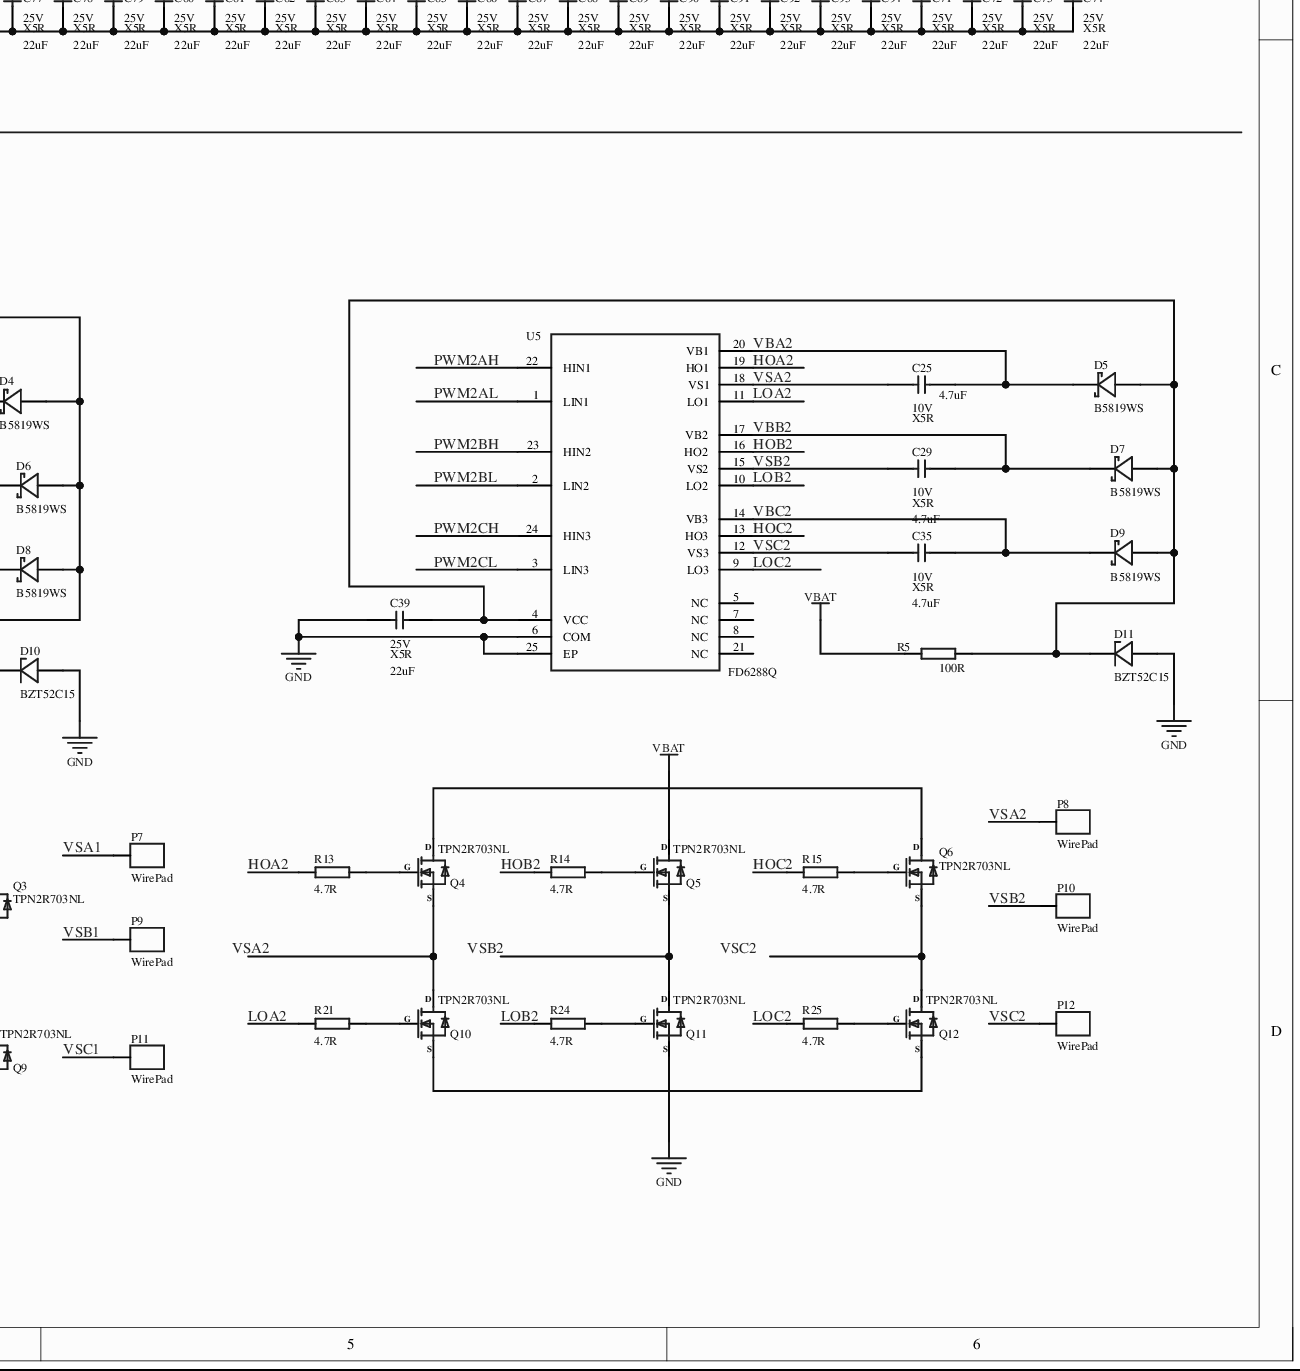
[diagram p0: MISC49862-3.schdoc, bottom right]
# Altium project MISC49862-2.PrjPcb (part 4 of 4)

## Sheet MISC49862-3.schdoc (continued)

### Library data of the parts (continued)
R9 = =Value+' '+Tolerance: SMD resistor; Device: 100R ±1%; Symbol: Res-Chip; Tolerance: ±1%; Origin Footprint 2: RESC0603[0201]-L; Origin Footprint 3: RESC0603[0201]-M; Origin Footprint 4: RESC0603[0201]-N; Origin Footprint 5: RESC0603[0201]S-L; Origin Footprint 6: RESC0603[0201]S-M; Origin Footprint 7: RESC0603[0201]S-N; Origin Footprint 8: RESC1005[0402]-L; Origin Footprint 9: RESC1005[0402]-M; Origin Footprint 10: RESC1005[0402]-N; Origin Footprint 11: RESC1005[0402]S-L; Origin Footprint 12: RESC1005[0402]S-M; Origin Footprint 13: RESC1608[0603]-L; Origin Footprint 14: RESC1608[0603]-M; Origin Footprint 15: RESC1608[0603]-N; Origin Footprint 16: RESC1608[0603]S-L; Origin Footprint 17: RESC1608[0603]S-M; Origin Footprint 18: RESC1608[0603]S-N; Origin Footprint 19: RESC2012[0805]; Origin Footprint 20: RESC2012[0805]S-L; Origin Footprint 21: RESC2012[0805]S-M; Origin Footprint 22: RESC2012[0805]S-N; Origin Footprint 23: RESC3216[1206]; Origin Footprint 24: RESC3216[1206]S-L; Origin Footprint 25: RESC3216[1206]S-M; Origin Footprint 26: RESC3216[1206]S-N; Origin Footprint 27: RESC3225[1210]; Origin Footprint 28: RESC3225[1210]S; Origin Footprint 29: RESC5025[2010]; Origin Footprint 30: RESC5025[2010]S; Origin Footprint 31: RESC6332[2512]; Origin Footprint 32: RESC6332[2512]S; UniqueId: 1e1ffada38203b9e; AddInBom: yes; Origin Footprint 1: RESC1005[0402]S-N; Design Item ID: Res-Chip; Library Name: Brushless driver-CYT2BL3-FD6288-FOC-LiteDual; Revision: V1.0; FootprintName: RESC1005[0402]S-N; ConvertToPcb: yes
R10 = =Value+' '+Tolerance: SMD resistor; Device: 4.7K ±1%; Symbol: Res-Chip_4; Tolerance: ±1%; Origin Footprint 2: RESC0603[0201]-L; Origin Footprint 3: RESC0603[0201]-M; Origin Footprint 4: RESC0603[0201]-N; Origin Footprint 5: RESC0603[0201]S-L; Origin Footprint 6: RESC0603[0201]S-M; Origin Footprint 7: RESC0603[0201]S-N; Origin Footprint 8: RESC1005[0402]-L; Origin Footprint 9: RESC1005[0402]-M; Origin Footprint 10: RESC1005[0402]-N; Origin Footprint 11: RESC1005[0402]S-L; Origin Footprint 12: RESC1005[0402]S-M; Origin Footprint 13: RESC1608[0603]-L; Origin Footprint 14: RESC1608[0603]-M; Origin Footprint 15: RESC1608[0603]-N; Origin Footprint 16: RESC1608[0603]S-L; Origin Footprint 17: RESC1608[0603]S-M; Origin Footprint 18: RESC1608[0603]S-N; Origin Footprint 19: RESC2012[0805]; Origin Footprint 20: RESC2012[0805]S-L; Origin Footprint 21: RESC2012[0805]S-M; Origin Footprint 22: RESC2012[0805]S-N; Origin Footprint 23: RESC3216[1206]; Origin Footprint 24: RESC3216[1206]S-L; Origin Footprint 25: RESC3216[1206]S-M; Origin Footprint 26: RESC3216[1206]S-N; Origin Footprint 27: RESC3225[1210]; Origin Footprint 28: RESC3225[1210]S; Origin Footprint 29: RESC5025[2010]; Origin Footprint 30: RESC5025[2010]S; Origin Footprint 31: RESC6332[2512]; Origin Footprint 32: RESC6332[2512]S; UniqueId: 41bc0941336b1513; AddInBom: yes; Origin Footprint 1: RESC1005[0402]S-N; Design Item ID: Res-Chip_4; Library Name: Brushless driver-CYT2BL3-FD6288-FOC-LiteDual; Revision: V1.0; FootprintName: RESC1005[0402]S-N; ConvertToPcb: yes
R11 = =Value+' '+Tolerance: SMD resistor; Device: 4.7R ±1%; Symbol: Res-Chip_7; Tolerance: ±1%; Origin Footprint 2: RESC0603[0201]-L; Origin Footprint 3: RESC0603[0201]-M; Origin Footprint 4: RESC0603[0201]-N; Origin Footprint 5: RESC0603[0201]S-L; Origin Footprint 6: RESC0603[0201]S-M; Origin Footprint 7: RESC0603[0201]S-N; Origin Footprint 8: RESC1005[0402]-L; Origin Footprint 9: RESC1005[0402]-M; Origin Footprint 10: RESC1005[0402]-N; Origin Footprint 11: RESC1005[0402]S-L; Origin Footprint 12: RESC1005[0402]S-M; Origin Footprint 13: RESC1608[0603]-L; Origin Footprint 14: RESC1608[0603]-M; Origin Footprint 15: RESC1608[0603]-N; Origin Footprint 16: RESC1608[0603]S-L; Origin Footprint 17: RESC1608[0603]S-M; Origin Footprint 18: RESC1608[0603]S-N; Origin Footprint 19: RESC2012[0805]; Origin Footprint 20: RESC2012[0805]S-L; Origin Footprint 21: RESC2012[0805]S-M; Origin Footprint 22: RESC2012[0805]S-N; Origin Footprint 23: RESC3216[1206]; Origin Footprint 24: RESC3216[1206]S-L; Origin Footprint 25: RESC3216[1206]S-M; Origin Footprint 26: RESC3216[1206]S-N; Origin Footprint 27: RESC3225[1210]; Origin Footprint 28: RESC3225[1210]S; Origin Footprint 29: RESC5025[2010]; Origin Footprint 30: RESC5025[2010]S; Origin Footprint 31: RESC6332[2512]; Origin Footprint 32: RESC6332[2512]S; UniqueId: 763cf8d5648cb4fd; AddInBom: yes; Origin Footprint 1: RESC1005[0402]S-N; Design Item ID: Res-Chip; Library Name: SEEKFREE_Device; Revision: V1.0; FootprintName: RESC1005[0402]S-N; ConvertToPcb: yes
R12 = =Value+' '+Tolerance: SMD resistor; Device: 1K ±1%; Symbol: Res-Chip_3; Tolerance: ±1%; Origin Footprint 2: RESC0603[0201]-L; Origin Footprint 3: RESC0603[0201]-M; Origin Footprint 4: RESC0603[0201]-N; Origin Footprint 5: RESC0603[0201]S-L; Origin Footprint 6: RESC0603[0201]S-M; Origin Footprint 7: RESC0603[0201]S-N; Origin Footprint 8: RESC1005[0402]-L; Origin Footprint 9: RESC1005[0402]-M; Origin Footprint 10: RESC1005[0402]-N; Origin Footprint 11: RESC1005[0402]S-L; Origin Footprint 12: RESC1005[0402]S-M; Origin Footprint 13: RESC1608[0603]-L; Origin Footprint 14: RESC1608[0603]-M; Origin Footprint 15: RESC1608[0603]-N; Origin Footprint 16: RESC1608[0603]S-L; Origin Footprint 17: RESC1608[0603]S-M; Origin Footprint 18: RESC1608[0603]S-N; Origin Footprint 19: RESC2012[0805]; Origin Footprint 20: RESC2012[0805]S-L; Origin Footprint 21: RESC2012[0805]S-M; Origin Footprint 22: RESC2012[0805]S-N; Origin Footprint 23: RESC3216[1206]; Origin Footprint 24: RESC3216[1206]S-L; Origin Footprint 25: RESC3216[1206]S-M; Origin Footprint 26: RESC3216[1206]S-N; Origin Footprint 27: RESC3225[1210]; Origin Footprint 28: RESC3225[1210]S; Origin Footprint 29: RESC5025[2010]; Origin Footprint 30: RESC5025[2010]S; Origin Footprint 31: RESC6332[2512]; Origin Footprint 32: RESC6332[2512]S; UniqueId: 15ac9218146e0f4b; AddInBom: yes; Origin Footprint 1: RESC1005[0402]S-N; Design Item ID: Res-Chip_3; Library Name: Brushless driver-CYT2BL3-FD6288-FOC-LiteDual; Revision: V1.0; FootprintName: RESC1005[0402]S-N; ConvertToPcb: yes
R13 = =Value+' '+Tolerance: SMD resistor; Device: 4.7R ±1%; Symbol: Res-Chip_7; Tolerance: ±1%; Origin Footprint 2: RESC0603[0201]-L; Origin Footprint 3: RESC0603[0201]-M; Origin Footprint 4: RESC0603[0201]-N; Origin Footprint 5: RESC0603[0201]S-L; Origin Footprint 6: RESC0603[0201]S-M; Origin Footprint 7: RESC0603[0201]S-N; Origin Footprint 8: RESC1005[0402]-L; Origin Footprint 9: RESC1005[0402]-M; Origin Footprint 10: RESC1005[0402]-N; Origin Footprint 11: RESC1005[0402]S-L; Origin Footprint 12: RESC1005[0402]S-M; Origin Footprint 13: RESC1608[0603]-L; Origin Footprint 14: RESC1608[0603]-M; Origin Footprint 15: RESC1608[0603]-N; Origin Footprint 16: RESC1608[0603]S-L; Origin Footprint 17: RESC1608[0603]S-M; Origin Footprint 18: RESC1608[0603]S-N; Origin Footprint 19: RESC2012[0805]; Origin Footprint 20: RESC2012[0805]S-L; Origin Footprint 21: RESC2012[0805]S-M; Origin Footprint 22: RESC2012[0805]S-N; Origin Footprint 23: RESC3216[1206]; Origin Footprint 24: RESC3216[1206]S-L; Origin Footprint 25: RESC3216[1206]S-M; Origin Footprint 26: RESC3216[1206]S-N; Origin Footprint 27: RESC3225[1210]; Origin Footprint 28: RESC3225[1210]S; Origin Footprint 29: RESC5025[2010]; Origin Footprint 30: RESC5025[2010]S; Origin Footprint 31: RESC6332[2512]; Origin Footprint 32: RESC6332[2512]S; UniqueId: ff4077a9ca69db92; AddInBom: yes; Origin Footprint 1: RESC1005[0402]S-N; Design Item ID: Res-Chip; Library Name: SEEKFREE_Device; Revision: V1.0; FootprintName: RESC1005[0402]S-N; ConvertToPcb: yes
R14 = =Value+' '+Tolerance: SMD resistor; Device: 4.7R ±1%; Symbol: Res-Chip_7; Tolerance: ±1%; Origin Footprint 2: RESC0603[0201]-L; Origin Footprint 3: RESC0603[0201]-M; Origin Footprint 4: RESC0603[0201]-N; Origin Footprint 5: RESC0603[0201]S-L; Origin Footprint 6: RESC0603[0201]S-M; Origin Footprint 7: RESC0603[0201]S-N; Origin Footprint 8: RESC1005[0402]-L; Origin Footprint 9: RESC1005[0402]-M; Origin Footprint 10: RESC1005[0402]-N; Origin Footprint 11: RESC1005[0402]S-L; Origin Footprint 12: RESC1005[0402]S-M; Origin Footprint 13: RESC1608[0603]-L; Origin Footprint 14: RESC1608[0603]-M; Origin Footprint 15: RESC1608[0603]-N; Origin Footprint 16: RESC1608[0603]S-L; Origin Footprint 17: RESC1608[0603]S-M; Origin Footprint 18: RESC1608[0603]S-N; Origin Footprint 19: RESC2012[0805]; Origin Footprint 20: RESC2012[0805]S-L; Origin Footprint 21: RESC2012[0805]S-M; Origin Footprint 22: RESC2012[0805]S-N; Origin Footprint 23: RESC3216[1206]; Origin Footprint 24: RESC3216[1206]S-L; Origin Footprint 25: RESC3216[1206]S-M; Origin Footprint 26: RESC3216[1206]S-N; Origin Footprint 27: RESC3225[1210]; Origin Footprint 28: RESC3225[1210]S; Origin Footprint 29: RESC5025[2010]; Origin Footprint 30: RESC5025[2010]S; Origin Footprint 31: RESC6332[2512]; Origin Footprint 32: RESC6332[2512]S; UniqueId: 8b54177fc4d64d35; AddInBom: yes; Origin Footprint 1: RESC1005[0402]S-N; Design Item ID: Res-Chip; Library Name: SEEKFREE_Device; Revision: V1.0; FootprintName: RESC1005[0402]S-N; ConvertToPcb: yes
R15 = =Value+' '+Tolerance: SMD resistor; Device: 4.7R ±1%; Symbol: Res-Chip_7; Tolerance: ±1%; Origin Footprint 2: RESC0603[0201]-L; Origin Footprint 3: RESC0603[0201]-M; Origin Footprint 4: RESC0603[0201]-N; Origin Footprint 5: RESC0603[0201]S-L; Origin Footprint 6: RESC0603[0201]S-M; Origin Footprint 7: RESC0603[0201]S-N; Origin Footprint 8: RESC1005[0402]-L; Origin Footprint 9: RESC1005[0402]-M; Origin Footprint 10: RESC1005[0402]-N; Origin Footprint 11: RESC1005[0402]S-L; Origin Footprint 12: RESC1005[0402]S-M; Origin Footprint 13: RESC1608[0603]-L; Origin Footprint 14: RESC1608[0603]-M; Origin Footprint 15: RESC1608[0603]-N; Origin Footprint 16: RESC1608[0603]S-L; Origin Footprint 17: RESC1608[0603]S-M; Origin Footprint 18: RESC1608[0603]S-N; Origin Footprint 19: RESC2012[0805]; Origin Footprint 20: RESC2012[0805]S-L; Origin Footprint 21: RESC2012[0805]S-M; Origin Footprint 22: RESC2012[0805]S-N; Origin Footprint 23: RESC3216[1206]; Origin Footprint 24: RESC3216[1206]S-L; Origin Footprint 25: RESC3216[1206]S-M; Origin Footprint 26: RESC3216[1206]S-N; Origin Footprint 27: RESC3225[1210]; Origin Footprint 28: RESC3225[1210]S; Origin Footprint 29: RESC5025[2010]; Origin Footprint 30: RESC5025[2010]S; Origin Footprint 31: RESC6332[2512]; Origin Footprint 32: RESC6332[2512]S; UniqueId: feece054417b9159; AddInBom: yes; Origin Footprint 1: RESC1005[0402]S-N; Design Item ID: Res-Chip; Library Name: SEEKFREE_Device; Revision: V1.0; FootprintName: RESC1005[0402]S-N; ConvertToPcb: yes
R16 = =Value+' '+Tolerance: SMD resistor; Device: 4.7R ±1%; Symbol: Res-Chip_7; Tolerance: ±1%; Origin Footprint 2: RESC0603[0201]-L; Origin Footprint 3: RESC0603[0201]-M; Origin Footprint 4: RESC0603[0201]-N; Origin Footprint 5: RESC0603[0201]S-L; Origin Footprint 6: RESC0603[0201]S-M; Origin Footprint 7: RESC0603[0201]S-N; Origin Footprint 8: RESC1005[0402]-L; Origin Footprint 9: RESC1005[0402]-M; Origin Footprint 10: RESC1005[0402]-N; Origin Footprint 11: RESC1005[0402]S-L; Origin Footprint 12: RESC1005[0402]S-M; Origin Footprint 13: RESC1608[0603]-L; Origin Footprint 14: RESC1608[0603]-M; Origin Footprint 15: RESC1608[0603]-N; Origin Footprint 16: RESC1608[0603]S-L; Origin Footprint 17: RESC1608[0603]S-M; Origin Footprint 18: RESC1608[0603]S-N; Origin Footprint 19: RESC2012[0805]; Origin Footprint 20: RESC2012[0805]S-L; Origin Footprint 21: RESC2012[0805]S-M; Origin Footprint 22: RESC2012[0805]S-N; Origin Footprint 23: RESC3216[1206]; Origin Footprint 24: RESC3216[1206]S-L; Origin Footprint 25: RESC3216[1206]S-M; Origin Footprint 26: RESC3216[1206]S-N; Origin Footprint 27: RESC3225[1210]; Origin Footprint 28: RESC3225[1210]S; Origin Footprint 29: RESC5025[2010]; Origin Footprint 30: RESC5025[2010]S; Origin Footprint 31: RESC6332[2512]; Origin Footprint 32: RESC6332[2512]S; UniqueId: 3c543c7c58e1cc80; AddInBom: yes; Origin Footprint 1: RESC1005[0402]S-N; Design Item ID: Res-Chip; Library Name: SEEKFREE_Device; Revision: V1.0; FootprintName: RESC1005[0402]S-N; ConvertToPcb: yes
R17 = =Value+' '+Tolerance: SMD resistor; Device: 1K ±1%; Symbol: Res-Chip_3; Tolerance: ±1%; Origin Footprint 2: RESC0603[0201]-L; Origin Footprint 3: RESC0603[0201]-M; Origin Footprint 4: RESC0603[0201]-N; Origin Footprint 5: RESC0603[0201]S-L; Origin Footprint 6: RESC0603[0201]S-M; Origin Footprint 7: RESC0603[0201]S-N; Origin Footprint 8: RESC1005[0402]-L; Origin Footprint 9: RESC1005[0402]-M; Origin Footprint 10: RESC1005[0402]-N; Origin Footprint 11: RESC1005[0402]S-L; Origin Footprint 12: RESC1005[0402]S-M; Origin Footprint 13: RESC1608[0603]-L; Origin Footprint 14: RESC1608[0603]-M; Origin Footprint 15: RESC1608[0603]-N; Origin Footprint 16: RESC1608[0603]S-L; Origin Footprint 17: RESC1608[0603]S-M; Origin Footprint 18: RESC1608[0603]S-N; Origin Footprint 19: RESC2012[0805]; Origin Footprint 20: RESC2012[0805]S-L; Origin Footprint 21: RESC2012[0805]S-M; Origin Footprint 22: RESC2012[0805]S-N; Origin Footprint 23: RESC3216[1206]; Origin Footprint 24: RESC3216[1206]S-L; Origin Footprint 25: RESC3216[1206]S-M; Origin Footprint 26: RESC3216[1206]S-N; Origin Footprint 27: RESC3225[1210]; Origin Footprint 28: RESC3225[1210]S; Origin Footprint 29: RESC5025[2010]; Origin Footprint 30: RESC5025[2010]S; Origin Footprint 31: RESC6332[2512]; Origin Footprint 32: RESC6332[2512]S; UniqueId: 6346d187b4e0bc9c; AddInBom: yes; Origin Footprint 1: RESC1005[0402]S-N; Design Item ID: Res-Chip_3; Library Name: Brushless driver-CYT2BL3-FD6288-FOC-LiteDual; Revision: V1.0; FootprintName: RESC1005[0402]S-N; ConvertToPcb: yes
R18 = =Value+' '+Tolerance: SMD resistor; Device: 4.7R ±1%; Symbol: Res-Chip_7; Tolerance: ±1%; Origin Footprint 2: RESC0603[0201]-L; Origin Footprint 3: RESC0603[0201]-M; Origin Footprint 4: RESC0603[0201]-N; Origin Footprint 5: RESC0603[0201]S-L; Origin Footprint 6: RESC0603[0201]S-M; Origin Footprint 7: RESC0603[0201]S-N; Origin Footprint 8: RESC1005[0402]-L; Origin Footprint 9: RESC1005[0402]-M; Origin Footprint 10: RESC1005[0402]-N; Origin Footprint 11: RESC1005[0402]S-L; Origin Footprint 12: RESC1005[0402]S-M; Origin Footprint 13: RESC1608[0603]-L; Origin Footprint 14: RESC1608[0603]-M; Origin Footprint 15: RESC1608[0603]-N; Origin Footprint 16: RESC1608[0603]S-L; Origin Footprint 17: RESC1608[0603]S-M; Origin Footprint 18: RESC1608[0603]S-N; Origin Footprint 19: RESC2012[0805]; Origin Footprint 20: RESC2012[0805]S-L; Origin Footprint 21: RESC2012[0805]S-M; Origin Footprint 22: RESC2012[0805]S-N; Origin Footprint 23: RESC3216[1206]; Origin Footprint 24: RESC3216[1206]S-L; Origin Footprint 25: RESC3216[1206]S-M; Origin Footprint 26: RESC3216[1206]S-N; Origin Footprint 27: RESC3225[1210]; Origin Footprint 28: RESC3225[1210]S; Origin Footprint 29: RESC5025[2010]; Origin Footprint 30: RESC5025[2010]S; Origin Footprint 31: RESC6332[2512]; Origin Footprint 32: RESC6332[2512]S; UniqueId: 5f673669f0d56d8f; AddInBom: yes; Origin Footprint 1: RESC1005[0402]S-N; Design Item ID: Res-Chip; Library Name: SEEKFREE_Device; Revision: V1.0; FootprintName: RESC1005[0402]S-N; ConvertToPcb: yes
R19 = =Value+' '+Tolerance: SMD resistor; Device: 4.7R ±1%; Symbol: Res-Chip_7; Tolerance: ±1%; Origin Footprint 2: RESC0603[0201]-L; Origin Footprint 3: RESC0603[0201]-M; Origin Footprint 4: RESC0603[0201]-N; Origin Footprint 5: RESC0603[0201]S-L; Origin Footprint 6: RESC0603[0201]S-M; Origin Footprint 7: RESC0603[0201]S-N; Origin Footprint 8: RESC1005[0402]-L; Origin Footprint 9: RESC1005[0402]-M; Origin Footprint 10: RESC1005[0402]-N; Origin Footprint 11: RESC1005[0402]S-L; Origin Footprint 12: RESC1005[0402]S-M; Origin Footprint 13: RESC1608[0603]-L; Origin Footprint 14: RESC1608[0603]-M; Origin Footprint 15: RESC1608[0603]-N; Origin Footprint 16: RESC1608[0603]S-L; Origin Footprint 17: RESC1608[0603]S-M; Origin Footprint 18: RESC1608[0603]S-N; Origin Footprint 19: RESC2012[0805]; Origin Footprint 20: RESC2012[0805]S-L; Origin Footprint 21: RESC2012[0805]S-M; Origin Footprint 22: RESC2012[0805]S-N; Origin Footprint 23: RESC3216[1206]; Origin Footprint 24: RESC3216[1206]S-L; Origin Footprint 25: RESC3216[1206]S-M; Origin Footprint 26: RESC3216[1206]S-N; Origin Footprint 27: RESC3225[1210]; Origin Footprint 28: RESC3225[1210]S; Origin Footprint 29: RESC5025[2010]; Origin Footprint 30: RESC5025[2010]S; Origin Footprint 31: RESC6332[2512]; Origin Footprint 32: RESC6332[2512]S; UniqueId: a32210a39874d8f8; AddInBom: yes; Origin Footprint 1: RESC1005[0402]S-N; Design Item ID: Res-Chip; Library Name: SEEKFREE_Device; Revision: V1.0; FootprintName: RESC1005[0402]S-N; ConvertToPcb: yes
R20 = =Value+' '+Tolerance: SMD resistor; Device: 100R ±1%; Symbol: Res-Chip; Tolerance: ±1%; Origin Footprint 2: RESC0603[0201]-L; Origin Footprint 3: RESC0603[0201]-M; Origin Footprint 4: RESC0603[0201]-N; Origin Footprint 5: RESC0603[0201]S-L; Origin Footprint 6: RESC0603[0201]S-M; Origin Footprint 7: RESC0603[0201]S-N; Origin Footprint 8: RESC1005[0402]-L; Origin Footprint 9: RESC1005[0402]-M; Origin Footprint 10: RESC1005[0402]-N; Origin Footprint 11: RESC1005[0402]S-L; Origin Footprint 12: RESC1005[0402]S-M; Origin Footprint 13: RESC1608[0603]-L; Origin Footprint 14: RESC1608[0603]-M; Origin Footprint 15: RESC1608[0603]-N; Origin Footprint 16: RESC1608[0603]S-L; Origin Footprint 17: RESC1608[0603]S-M; Origin Footprint 18: RESC1608[0603]S-N; Origin Footprint 19: RESC2012[0805]; Origin Footprint 20: RESC2012[0805]S-L; Origin Footprint 21: RESC2012[0805]S-M; Origin Footprint 22: RESC2012[0805]S-N; Origin Footprint 23: RESC3216[1206]; Origin Footprint 24: RESC3216[1206]S-L; Origin Footprint 25: RESC3216[1206]S-M; Origin Footprint 26: RESC3216[1206]S-N; Origin Footprint 27: RESC3225[1210]; Origin Footprint 28: RESC3225[1210]S; Origin Footprint 29: RESC5025[2010]; Origin Footprint 30: RESC5025[2010]S; Origin Footprint 31: RESC6332[2512]; Origin Footprint 32: RESC6332[2512]S; UniqueId: 13e77c54ede4b306; AddInBom: yes; Origin Footprint 1: RESC1005[0402]S-N; Design Item ID: Res-Chip; Library Name: Brushless driver-CYT2BL3-FD6288-FOC-LiteDual; Revision: V1.0; FootprintName: RESC1005[0402]S-N; ConvertToPcb: yes
R21 = =Value+' '+Tolerance: SMD resistor; Device: 4.7R ±1%; Symbol: Res-Chip_7; Tolerance: ±1%; Origin Footprint 2: RESC0603[0201]-L; Origin Footprint 3: RESC0603[0201]-M; Origin Footprint 4: RESC0603[0201]-N; Origin Footprint 5: RESC0603[0201]S-L; Origin Footprint 6: RESC0603[0201]S-M; Origin Footprint 7: RESC0603[0201]S-N; Origin Footprint 8: RESC1005[0402]-L; Origin Footprint 9: RESC1005[0402]-M; Origin Footprint 10: RESC1005[0402]-N; Origin Footprint 11: RESC1005[0402]S-L; Origin Footprint 12: RESC1005[0402]S-M; Origin Footprint 13: RESC1608[0603]-L; Origin Footprint 14: RESC1608[0603]-M; Origin Footprint 15: RESC1608[0603]-N; Origin Footprint 16: RESC1608[0603]S-L; Origin Footprint 17: RESC1608[0603]S-M; Origin Footprint 18: RESC1608[0603]S-N; Origin Footprint 19: RESC2012[0805]; Origin Footprint 20: RESC2012[0805]S-L; Origin Footprint 21: RESC2012[0805]S-M; Origin Footprint 22: RESC2012[0805]S-N; Origin Footprint 23: RESC3216[1206]; Origin Footprint 24: RESC3216[1206]S-L; Origin Footprint 25: RESC3216[1206]S-M; Origin Footprint 26: RESC3216[1206]S-N; Origin Footprint 27: RESC3225[1210]; Origin Footprint 28: RESC3225[1210]S; Origin Footprint 29: RESC5025[2010]; Origin Footprint 30: RESC5025[2010]S; Origin Footprint 31: RESC6332[2512]; Origin Footprint 32: RESC6332[2512]S; UniqueId: c77b08197b178948; AddInBom: yes; Origin Footprint 1: RESC1005[0402]S-N; Design Item ID: Res-Chip; Library Name: SEEKFREE_Device; Revision: V1.0; FootprintName: RESC1005[0402]S-N; ConvertToPcb: yes
R22 = =Value+' '+Tolerance: SMD resistor; Device: 73.2K ±1%; Symbol: Res-Chip_5; Power: 1/8W; Tolerance: ±1%; Origin Footprint 2: RESC0603[0201]-L; Origin Footprint 3: RESC0603[0201]-M; Origin Footprint 4: RESC0603[0201]-N; Origin Footprint 5: RESC0603[0201]S-L; Origin Footprint 6: RESC0603[0201]S-M; Origin Footprint 7: RESC0603[0201]S-N; Origin Footprint 8: RESC1005[0402]-L; Origin Footprint 9: RESC1005[0402]S-M; Origin Footprint 10: RESC1005[0402]-M; Origin Footprint 11: RESC1005[0402]-N; Origin Footprint 12: RESC1005[0402]S-L; Origin Footprint 13: RESC1608[0603]-L; Origin Footprint 14: RESC1608[0603]-M; Origin Footprint 15: RESC1608[0603]-N; Origin Footprint 16: RESC1608[0603]S-L; Origin Footprint 17: RESC1608[0603]S-M; Origin Footprint 18: RESC1608[0603]S-N; Origin Footprint 19: RESC2012[0805]; Origin Footprint 20: RESC2012[0805]S-L; Origin Footprint 21: RESC2012[0805]S-M; Origin Footprint 22: RESC2012[0805]S-N; Origin Footprint 23: RESC3216[1206]; Origin Footprint 24: RESC3216[1206]S-L; Origin Footprint 25: RESC3216[1206]S-M; Origin Footprint 26: RESC3216[1206]S-N; Origin Footprint 27: RESC3225[1210]; Origin Footprint 28: RESC3225[1210]S; Origin Footprint 29: RESC5025[2010]; Origin Footprint 30: RESC5025[2010]S; Origin Footprint 31: RESC6332[2512]; Origin Footprint 32: RESC6332[2512]S; UniqueId: fa394caafc8878d8; AddInBom: yes; Origin Footprint 1: RESC1005[0402]S-N; Design Item ID: Res-Chip_5; Library Name: Brushless driver-CYT2BL3-FD6288-FOC-LiteDual; Revision: V1.0; FootprintName: RESC1005[0402]S-N; ConvertToPcb: yes
R23 = =Value+' '+Tolerance: SMD resistor; Device: 10K ±1%; Symbol: Res-Chip_1; Tolerance: ±1%; Origin Footprint 2: RESC0603[0201]-L; Origin Footprint 3: RESC0603[0201]-M; Origin Footprint 4: RESC0603[0201]-N; Origin Footprint 5: RESC0603[0201]S-L; Origin Footprint 6: RESC0603[0201]S-M; Origin Footprint 7: RESC0603[0201]S-N; Origin Footprint 8: RESC1005[0402]-L; Origin Footprint 9: RESC1005[0402]-M; Origin Footprint 10: RESC1005[0402]-N; Origin Footprint 11: RESC1005[0402]S-L; Origin Footprint 12: RESC1005[0402]S-M; Origin Footprint 13: RESC1608[0603]-L; Origin Footprint 14: RESC1608[0603]-M; Origin Footprint 15: RESC1608[0603]-N; Origin Footprint 16: RESC1608[0603]S-L; Origin Footprint 17: RESC1608[0603]S-M; Origin Footprint 18: RESC1608[0603]S-N; Origin Footprint 19: RESC2012[0805]; Origin Footprint 20: RESC2012[0805]S-L; Origin Footprint 21: RESC2012[0805]S-M; Origin Footprint 22: RESC2012[0805]S-N; Origin Footprint 23: RESC3216[1206]; Origin Footprint 24: RESC3216[1206]S-L; Origin Footprint 25: RESC3216[1206]S-M; Origin Footprint 26: RESC3216[1206]S-N; Origin Footprint 27: RESC3225[1210]; Origin Footprint 28: RESC3225[1210]S; Origin Footprint 29: RESC5025[2010]; Origin Footprint 30: RESC5025[2010]S; Origin Footprint 31: RESC6332[2512]; Origin Footprint 32: RESC6332[2512]S; UniqueId: d92c635076b33213; AddInBom: yes; Origin Footprint 1: RESC1005[0402]S-N; Design Item ID: Res-Chip_1; Library Name: Brushless driver-CYT2BL3-FD6288-FOC-LiteDual; Revision: V1.0; FootprintName: RESC1005[0402]S-N; ConvertToPcb: yes
R24 = =Value+' '+Tolerance: SMD resistor; Device: 4.7R ±1%; Symbol: Res-Chip_7; Tolerance: ±1%; Origin Footprint 2: RESC0603[0201]-L; Origin Footprint 3: RESC0603[0201]-M; Origin Footprint 4: RESC0603[0201]-N; Origin Footprint 5: RESC0603[0201]S-L; Origin Footprint 6: RESC0603[0201]S-M; Origin Footprint 7: RESC0603[0201]S-N; Origin Footprint 8: RESC1005[0402]-L; Origin Footprint 9: RESC1005[0402]-M; Origin Footprint 10: RESC1005[0402]-N; Origin Footprint 11: RESC1005[0402]S-L; Origin Footprint 12: RESC1005[0402]S-M; Origin Footprint 13: RESC1608[0603]-L; Origin Footprint 14: RESC1608[0603]-M; Origin Footprint 15: RESC1608[0603]-N; Origin Footprint 16: RESC1608[0603]S-L; Origin Footprint 17: RESC1608[0603]S-M; Origin Footprint 18: RESC1608[0603]S-N; Origin Footprint 19: RESC2012[0805]; Origin Footprint 20: RESC2012[0805]S-L; Origin Footprint 21: RESC2012[0805]S-M; Origin Footprint 22: RESC2012[0805]S-N; Origin Footprint 23: RESC3216[1206]; Origin Footprint 24: RESC3216[1206]S-L; Origin Footprint 25: RESC3216[1206]S-M; Origin Footprint 26: RESC3216[1206]S-N; Origin Footprint 27: RESC3225[1210]; Origin Footprint 28: RESC3225[1210]S; Origin Footprint 29: RESC5025[2010]; Origin Footprint 30: RESC5025[2010]S; Origin Footprint 31: RESC6332[2512]; Origin Footprint 32: RESC6332[2512]S; UniqueId: f7952e9f9cd6773b; AddInBom: yes; Origin Footprint 1: RESC1005[0402]S-N; Design Item ID: Res-Chip; Library Name: SEEKFREE_Device; Revision: V1.0; FootprintName: RESC1005[0402]S-N; ConvertToPcb: yes
R25 = =Value+' '+Tolerance: SMD resistor; Device: 4.7R ±1%; Symbol: Res-Chip_7; Tolerance: ±1%; Origin Footprint 2: RESC0603[0201]-L; Origin Footprint 3: RESC0603[0201]-M; Origin Footprint 4: RESC0603[0201]-N; Origin Footprint 5: RESC0603[0201]S-L; Origin Footprint 6: RESC0603[0201]S-M; Origin Footprint 7: RESC0603[0201]S-N; Origin Footprint 8: RESC1005[0402]-L; Origin Footprint 9: RESC1005[0402]-M; Origin Footprint 10: RESC1005[0402]-N; Origin Footprint 11: RESC1005[0402]S-L; Origin Footprint 12: RESC1005[0402]S-M; Origin Footprint 13: RESC1608[0603]-L; Origin Footprint 14: RESC1608[0603]-M; Origin Footprint 15: RESC1608[0603]-N; Origin Footprint 16: RESC1608[0603]S-L; Origin Footprint 17: RESC1608[0603]S-M; Origin Footprint 18: RESC1608[0603]S-N; Origin Footprint 19: RESC2012[0805]; Origin Footprint 20: RESC2012[0805]S-L; Origin Footprint 21: RESC2012[0805]S-M; Origin Footprint 22: RESC2012[0805]S-N; Origin Footprint 23: RESC3216[1206]; Origin Footprint 24: RESC3216[1206]S-L; Origin Footprint 25: RESC3216[1206]S-M; Origin Footprint 26: RESC3216[1206]S-N; Origin Footprint 27: RESC3225[1210]; Origin Footprint 28: RESC3225[1210]S; Origin Footprint 29: RESC5025[2010]; Origin Footprint 30: RESC5025[2010]S; Origin Footprint 31: RESC6332[2512]; Origin Footprint 32: RESC6332[2512]S; UniqueId: 6f4c4beafd605d3e; AddInBom: yes; Origin Footprint 1: RESC1005[0402]S-N; Design Item ID: Res-Chip; Library Name: SEEKFREE_Device; Revision: V1.0; FootprintName: RESC1005[0402]S-N; ConvertToPcb: yes
R26 = =Value+' '+Tolerance: SMD resistor; Device: 100R ±1%; Symbol: Res-Chip; Tolerance: ±1%; Origin Footprint 2: RESC0603[0201]-L; Origin Footprint 3: RESC0603[0201]-M; Origin Footprint 4: RESC0603[0201]-N; Origin Footprint 5: RESC0603[0201]S-L; Origin Footprint 6: RESC0603[0201]S-M; Origin Footprint 7: RESC0603[0201]S-N; Origin Footprint 8: RESC1005[0402]-L; Origin Footprint 9: RESC1005[0402]-M; Origin Footprint 10: RESC1005[0402]-N; Origin Footprint 11: RESC1005[0402]S-L; Origin Footprint 12: RESC1005[0402]S-M; Origin Footprint 13: RESC1608[0603]-L; Origin Footprint 14: RESC1608[0603]-M; Origin Footprint 15: RESC1608[0603]-N; Origin Footprint 16: RESC1608[0603]S-L; Origin Footprint 17: RESC1608[0603]S-M; Origin Footprint 18: RESC1608[0603]S-N; Origin Footprint 19: RESC2012[0805]; Origin Footprint 20: RESC2012[0805]S-L; Origin Footprint 21: RESC2012[0805]S-M; Origin Footprint 22: RESC2012[0805]S-N; Origin Footprint 23: RESC3216[1206]; Origin Footprint 24: RESC3216[1206]S-L; Origin Footprint 25: RESC3216[1206]S-M; Origin Footprint 26: RESC3216[1206]S-N; Origin Footprint 27: RESC3225[1210]; Origin Footprint 28: RESC3225[1210]S; Origin Footprint 29: RESC5025[2010]; Origin Footprint 30: RESC5025[2010]S; Origin Footprint 31: RESC6332[2512]; Origin Footprint 32: RESC6332[2512]S; UniqueId: 09b823a69019dbbf; AddInBom: yes; Origin Footprint 1: RESC1005[0402]S-N; Design Item ID: Res-Chip; Library Name: Brushless driver-CYT2BL3-FD6288-FOC-LiteDual; Revision: V1.0; FootprintName: RESC1005[0402]S-N; ConvertToPcb: yes
R38 = =Value+' '+Tolerance: SMD resistor; Device: 45.3K ±1%; Symbol: Res-Chip_6; Power: 1/8W; Tolerance: ±1%; Origin Footprint 2: RESC0603[0201]-L; Origin Footprint 3: RESC0603[0201]-M; Origin Footprint 4: RESC0603[0201]-N; Origin Footprint 5: RESC0603[0201]S-L; Origin Footprint 6: RESC0603[0201]S-M; Origin Footprint 7: RESC0603[0201]S-N; Origin Footprint 8: RESC1005[0402]-L; Origin Footprint 9: RESC1005[0402]S-M; Origin Footprint 10: RESC1005[0402]-M; Origin Footprint 11: RESC1005[0402]-N; Origin Footprint 12: RESC1005[0402]S-L; Origin Footprint 13: RESC1608[0603]-L; Origin Footprint 14: RESC1608[0603]-M; Origin Footprint 15: RESC1608[0603]-N; Origin Footprint 16: RESC1608[0603]S-L; Origin Footprint 17: RESC1608[0603]S-M; Origin Footprint 18: RESC1608[0603]S-N; Origin Footprint 19: RESC2012[0805]; Origin Footprint 20: RESC2012[0805]S-L; Origin Footprint 21: RESC2012[0805]S-M; Origin Footprint 22: RESC2012[0805]S-N; Origin Footprint 23: RESC3216[1206]; Origin Footprint 24: RESC3216[1206]S-L; Origin Footprint 25: RESC3216[1206]S-M; Origin Footprint 26: RESC3216[1206]S-N; Origin Footprint 27: RESC3225[1210]; Origin Footprint 28: RESC3225[1210]S; Origin Footprint 29: RESC5025[2010]; Origin Footprint 30: RESC5025[2010]S; Origin Footprint 31: RESC6332[2512]; Origin Footprint 32: RESC6332[2512]S; UniqueId: 2eb3813281b987ab; AddInBom: yes; Origin Footprint 1: RESC1005[0402]S-N; Design Item ID: Res-Chip_6; Library Name: Brushless driver-CYT2BL3-FD6288-FOC-LiteDual; Revision: V1.0; FootprintName: RESC1005[0402]S-N; ConvertToPcb: yes
R45 = =Value+' '+Tolerance: SMD resistor; Device: 10K ±1%; Symbol: Res-Chip_1; Tolerance: ±1%; Origin Footprint 2: RESC0603[0201]-L; Origin Footprint 3: RESC0603[0201]-M; Origin Footprint 4: RESC0603[0201]-N; Origin Footprint 5: RESC0603[0201]S-L; Origin Footprint 6: RESC0603[0201]S-M; Origin Footprint 7: RESC0603[0201]S-N; Origin Footprint 8: RESC1005[0402]-L; Origin Footprint 9: RESC1005[0402]-M; Origin Footprint 10: RESC1005[0402]-N; Origin Footprint 11: RESC1005[0402]S-L; Origin Footprint 12: RESC1005[0402]S-M; Origin Footprint 13: RESC1608[0603]-L; Origin Footprint 14: RESC1608[0603]-M; Origin Footprint 15: RESC1608[0603]-N; Origin Footprint 16: RESC1608[0603]S-L; Origin Footprint 17: RESC1608[0603]S-M; Origin Footprint 18: RESC1608[0603]S-N; Origin Footprint 19: RESC2012[0805]; Origin Footprint 20: RESC2012[0805]S-L; Origin Footprint 21: RESC2012[0805]S-M; Origin Footprint 22: RESC2012[0805]S-N; Origin Footprint 23: RESC3216[1206]; Origin Footprint 24: RESC3216[1206]S-L; Origin Footprint 25: RESC3216[1206]S-M; Origin Footprint 26: RESC3216[1206]S-N; Origin Footprint 27: RESC3225[1210]; Origin Footprint 28: RESC3225[1210]S; Origin Footprint 29: RESC5025[2010]; Origin Footprint 30: RESC5025[2010]S; Origin Footprint 31: RESC6332[2512]; Origin Footprint 32: RESC6332[2512]S; UniqueId: fe3640da4f52432f; AddInBom: yes; Origin Footprint 1: RESC1005[0402]S-N; Design Item ID: Res-Chip_1; Library Name: Brushless driver-CYT2BL3-FD6288-FOC-LiteDual; Revision: V1.0; FootprintName: RESC1005[0402]S-N; ConvertToPcb: yes
R68 = =Value+' '+Tolerance: SMD resistor; Device: 1K ±1%; Symbol: Res-Chip_3; Tolerance: ±1%; Origin Footprint 2: RESC0603[0201]-L; Origin Footprint 3: RESC0603[0201]-M; Origin Footprint 4: RESC0603[0201]-N; Origin Footprint 5: RESC0603[0201]S-L; Origin Footprint 6: RESC0603[0201]S-M; Origin Footprint 7: RESC0603[0201]S-N; Origin Footprint 8: RESC1005[0402]-L; Origin Footprint 9: RESC1005[0402]-M; Origin Footprint 10: RESC1005[0402]-N; Origin Footprint 11: RESC1005[0402]S-L; Origin Footprint 12: RESC1005[0402]S-M; Origin Footprint 13: RESC1608[0603]-L; Origin Footprint 14: RESC1608[0603]-M; Origin Footprint 15: RESC1608[0603]-N; Origin Footprint 16: RESC1608[0603]S-L; Origin Footprint 17: RESC1608[0603]S-M; Origin Footprint 18: RESC1608[0603]S-N; Origin Footprint 19: RESC2012[0805]; Origin Footprint 20: RESC2012[0805]S-L; Origin Footprint 21: RESC2012[0805]S-M; Origin Footprint 22: RESC2012[0805]S-N; Origin Footprint 23: RESC3216[1206]; Origin Footprint 24: RESC3216[1206]S-L; Origin Footprint 25: RESC3216[1206]S-M; Origin Footprint 26: RESC3216[1206]S-N; Origin Footprint 27: RESC3225[1210]; Origin Footprint 28: RESC3225[1210]S; Origin Footprint 29: RESC5025[2010]; Origin Footprint 30: RESC5025[2010]S; Origin Footprint 31: RESC6332[2512]; Origin Footprint 32: RESC6332[2512]S; UniqueId: c6a558d5d37ead57; AddInBom: yes; Origin Footprint 1: RESC1005[0402]S-N; Design Item ID: Res-Chip_3; Library Name: Brushless driver-CYT2BL3-FD6288-FOC-LiteDual; Revision: V1.0; FootprintName: RESC1005[0402]S-N; ConvertToPcb: yes
R69 = =Value+' '+Tolerance: SMD resistor; Device: 10K ±1%; Symbol: Res-Chip_1; Tolerance: ±1%; Origin Footprint 2: RESC0603[0201]-L; Origin Footprint 3: RESC0603[0201]-M; Origin Footprint 4: RESC0603[0201]-N; Origin Footprint 5: RESC0603[0201]S-L; Origin Footprint 6: RESC0603[0201]S-M; Origin Footprint 7: RESC0603[0201]S-N; Origin Footprint 8: RESC1005[0402]-L; Origin Footprint 9: RESC1005[0402]-M; Origin Footprint 10: RESC1005[0402]-N; Origin Footprint 11: RESC1005[0402]S-L; Origin Footprint 12: RESC1005[0402]S-M; Origin Footprint 13: RESC1608[0603]-L; Origin Footprint 14: RESC1608[0603]-M; Origin Footprint 15: RESC1608[0603]-N; Origin Footprint 16: RESC1608[0603]S-L; Origin Footprint 17: RESC1608[0603]S-M; Origin Footprint 18: RESC1608[0603]S-N; Origin Footprint 19: RESC2012[0805]; Origin Footprint 20: RESC2012[0805]S-L; Origin Footprint 21: RESC2012[0805]S-M; Origin Footprint 22: RESC2012[0805]S-N; Origin Footprint 23: RESC3216[1206]; Origin Footprint 24: RESC3216[1206]S-L; Origin Footprint 25: RESC3216[1206]S-M; Origin Footprint 26: RESC3216[1206]S-N; Origin Footprint 27: RESC3225[1210]; Origin Footprint 28: RESC3225[1210]S; Origin Footprint 29: RESC5025[2010]; Origin Footprint 30: RESC5025[2010]S; Origin Footprint 31: RESC6332[2512]; Origin Footprint 32: RESC6332[2512]S; UniqueId: 8075c5db455eac63; AddInBom: yes; Origin Footprint 1: RESC1005[0402]S-N; Design Item ID: Res-Chip_1; Library Name: Brushless driver-CYT2BL3-FD6288-FOC-LiteDual; Revision: V1.0; FootprintName: RESC1005[0402]S-N; ConvertToPcb: yes
R70 = =Value+' '+Tolerance: SMD resistor; Device: 100R ±1%; Symbol: Res-Chip; Tolerance: ±1%; Origin Footprint 2: RESC0603[0201]-L; Origin Footprint 3: RESC0603[0201]-M; Origin Footprint 4: RESC0603[0201]-N; Origin Footprint 5: RESC0603[0201]S-L; Origin Footprint 6: RESC0603[0201]S-M; Origin Footprint 7: RESC0603[0201]S-N; Origin Footprint 8: RESC1005[0402]-L; Origin Footprint 9: RESC1005[0402]-M; Origin Footprint 10: RESC1005[0402]-N; Origin Footprint 11: RESC1005[0402]S-L; Origin Footprint 12: RESC1005[0402]S-M; Origin Footprint 13: RESC1608[0603]-L; Origin Footprint 14: RESC1608[0603]-M; Origin Footprint 15: RESC1608[0603]-N; Origin Footprint 16: RESC1608[0603]S-L; Origin Footprint 17: RESC1608[0603]S-M; Origin Footprint 18: RESC1608[0603]S-N; Origin Footprint 19: RESC2012[0805]; Origin Footprint 20: RESC2012[0805]S-L; Origin Footprint 21: RESC2012[0805]S-M; Origin Footprint 22: RESC2012[0805]S-N; Origin Footprint 23: RESC3216[1206]; Origin Footprint 24: RESC3216[1206]S-L; Origin Footprint 25: RESC3216[1206]S-M; Origin Footprint 26: RESC3216[1206]S-N; Origin Footprint 27: RESC3225[1210]; Origin Footprint 28: RESC3225[1210]S; Origin Footprint 29: RESC5025[2010]; Origin Footprint 30: RESC5025[2010]S; Origin Footprint 31: RESC6332[2512]; Origin Footprint 32: RESC6332[2512]S; UniqueId: 593bc9c00f33e5d7; AddInBom: yes; Origin Footprint 1: RESC1005[0402]S-N; Design Item ID: Res-Chip; Library Name: Brushless driver-CYT2BL3-FD6288-FOC-LiteDual; Revision: V1.0; FootprintName: RESC1005[0402]S-N; ConvertToPcb: yes
S1 = KEY-TS1145: 3x4x2.5 4-pin key SMD vertical press; Origin Footprint 2: TS1145-C-A; UniqueId: 0ac0bd892f9b1ec0; AddInBom: yes; Origin Footprint 1: TS1145-B-A; Device: KEY-TS1145; Symbol: KEY-TS1145; Design Item ID: KEY-TS1145; Library Name: Brushless driver-CYT2BL3-FD6288-FOC-LiteDual; Revision: V1.0; Value: KEY-TS1145; FootprintName: TS1145-B-A; ConvertToPcb: yes
S2 = KEY-TS1145: 3x4x2.5 4-pin key SMD vertical press; Origin Footprint 2: TS1145-C-A; UniqueId: 16ca49f37df57620; AddInBom: yes; Origin Footprint 1: TS1145-B-A; Device: KEY-TS1145; Symbol: KEY-TS1145; Design Item ID: KEY-TS1145; Library Name: Brushless driver-CYT2BL3-FD6288-FOC-LiteDual; Revision: V1.0; Value: KEY-TS1145; FootprintName: TS1145-B-A; ConvertToPcb: yes
U1 = CYT2BL3CAx: Origin Footprint 2: LQFP64_M; Origin Footprint 3: LQFP64_N; UniqueId: 1bdc0ab44f99f92d; AddInBom: yes; Origin Footprint 1: LQFP64_L; Device: CYT2BL3CAx; Symbol: CYT2BL3CAx; Design Item ID: CYT2BL3CAx; Library Name: Brushless driver-CYT2BL3-FD6288-FOC-LiteDual; Description: CYT2BL3CAx; FootprintName: LQFP64_L; ConvertToPcb: yes
U2 = FD6288Q: FD6288Q three-phase gate driver; Origin Footprint 2: QFN24-4x4; UniqueId: 48f0ae2437312dae; AddInBom: yes; Origin Footprint 1: QFN24-4x4-L; Device: FD6288Q; Symbol: FD6288Q; Design Item ID: FD6288Q; Library Name: SEEKFREE_Device; FootprintName: QFN24-4x4-L; ConvertToPcb: yes
U4 = RY9121E: 17V 2A 1.2MHz Synchronous Step-Down Regulator; UniqueId: bac468049775df37; AddInBom: yes; Origin Footprint: SOT-23-6; Device: RY9121E; Symbol: RY9121E; Design Item ID: RY9121E; Library Name: Brushless driver-CYT2BL3-FD6288-FOC-LiteDual; Revision: V1.0; Value: RY9121E; FootprintName: SOT-23-6; ConvertToPcb: yes
U5 = FD6288Q: FD6288Q three-phase gate driver; Origin Footprint 2: QFN24-4x4; UniqueId: adf583383e4d69d4; AddInBom: yes; Origin Footprint 1: QFN24-4x4-L; Device: FD6288Q; Symbol: FD6288Q; Design Item ID: FD6288Q; Library Name: SEEKFREE_Device; FootprintName: QFN24-4x4-L; ConvertToPcb: yes
U7 = RY9121E: 17V 2A 1.2MHz Synchronous Step-Down Regulator; UniqueId: 4ec783ed4741de1f; AddInBom: yes; Origin Footprint: SOT-23-6; Device: RY9121E; Symbol: RY9121E; Design Item ID: RY9121E; Library Name: Brushless driver-CYT2BL3-FD6288-FOC-LiteDual; Revision: V1.0; Value: RY9121E; FootprintName: SOT-23-6; ConvertToPcb: yes
Y1 = =Frequency+' '+Load_Capactiance: Four-pin passive crystal oscillator Crystal Oscillator; Device: 16MHz 20pF; Symbol: XTAL-4; Origin Footprint 2: X2016-4; Origin Footprint 3: X2520-4; UniqueId: 9790cc8ece124e27; AddInBom: yes; Origin Footprint 1: X3225-4; Design Item ID: XTAL-4; Library Name: Brushless driver-CYT2BL3-FD6288-FOC-LiteDual; Revision: V1.0; FootprintName: X3225-4; ConvertToPcb: yes